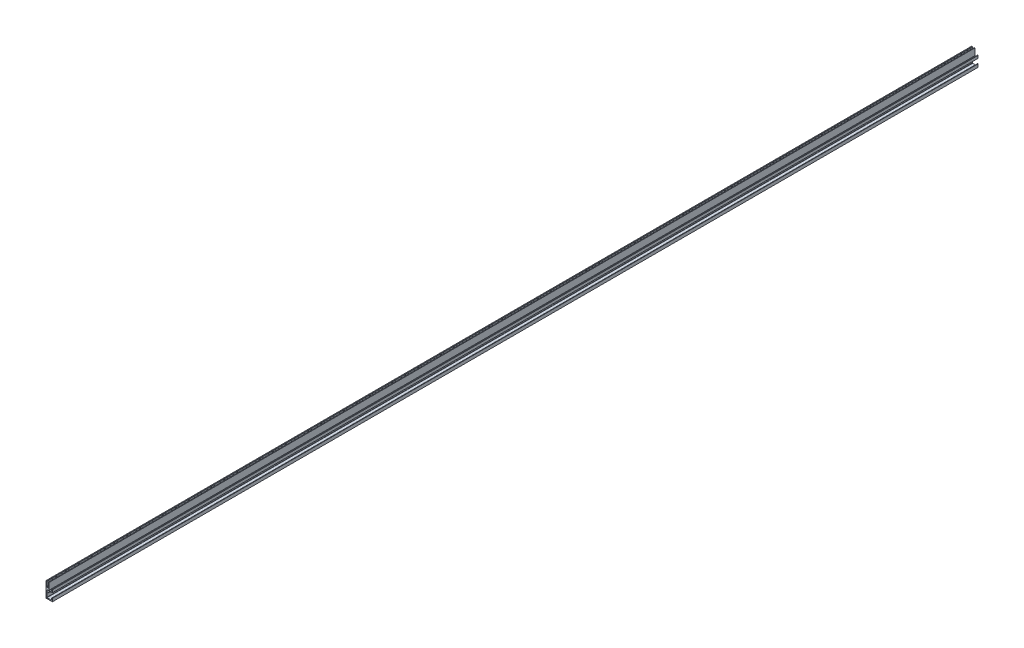
from build123d import *

# Parameters (mm, degrees)
EXTRUDE_1_DEPTH = 1058


with BuildPart() as part:
    # 草图2 → 凸台-拉伸1 (new, symmetric)
    with BuildSketch(Plane.XY):
        with BuildLine():
            Line((14.484958611, 7.149447031), (13.704975481, 7.149447031))
            ThreePointArc((13.704975481, 7.149447031), (13.280736974, 6.973721688), (13.105011631, 6.549483181))
            Line((13.105011631, 6.549483181), (13.105011631, 2.269839045))
            ThreePointArc((13.105011631, 2.269839045), (13.06986594, 2.184990722), (12.985017102, 2.149846275))
            Line((12.985017102, 2.149846275), (2.5, 2.15))
            ThreePointArc((2.5, 2.15), (2.146446609, 2.296446609), (2, 2.65))
            Line((2, 2.65), (2, 9.75))
            ThreePointArc((2, 9.75), (1.75, 10), (2, 10.25))
            Line((2, 10.25), (2, 17.35))
            ThreePointArc((2, 17.35), (2.146446609, 17.703553391), (2.5, 17.85))
            Line((2.5, 17.85), (14.604187277, 17.85))
            Line((14.604187277, 17.85), (14.604187277, 23.829737701))
            ThreePointArc((14.604187277, 23.829737701), (14.569042208, 23.914585402), (14.484194507, 23.949730471))
            Line((14.484194507, 23.949730471), (13.704211377, 23.949730471))
            ThreePointArc((13.704211377, 23.949730471), (13.27997287, 23.774005128), (13.104247527, 23.349766621))
            Line((13.104247527, 23.349766621), (13.104247527, 19.46999277))
            ThreePointArc((13.104247527, 19.46999277), (13.069102458, 19.385145069), (12.984254757, 19.35))
            Line((12.984254757, 19.35), (7.2, 19.35))
            Line((7.2, 19.35), (7.2, 34.798393128))
            Line((7.2, 34.798393128), (6, 34.798393128))
            ThreePointArc((6, 34.798393128), (5.858578644, 34.739814485), (5.8, 34.598393128))
            Line((5.8, 34.598393128), (5.8, 33.098393128))
            ThreePointArc((5.8, 33.098393128), (5.7, 32.998393128), (5.8, 32.898393128))
            Line((5.8, 32.898393128), (5.8, 23.812239282))
            ThreePointArc((5.8, 23.812239282), (5.507106781, 23.105132501), (4.8, 22.812239282))
            Line((4.8, 22.812239282), (2.8, 22.812239282))
            ThreePointArc((2.8, 22.812239282), (2.092893219, 23.105132501), (1.8, 23.812239282))
            Line((1.8, 23.812239282), (1.8, 32.898393128))
            ThreePointArc((1.8, 32.898393128), (1.9, 32.998393128), (1.8, 33.098393128))
            Line((1.8, 33.098393128), (1.8, 34.598393128))
            ThreePointArc((1.8, 34.598393128), (1.741421356, 34.739814485), (1.6, 34.798393128))
            Line((1.6, 34.798393128), (0, 34.798393128))
            Line((0, 34.798393128), (0, 0))
            Line((0, 0), (14.6, 0))
            Line((14.6, 0), (14.604951381, 7.029454261))
            ThreePointArc((14.604951381, 7.029454261), (14.569806312, 7.114301962), (14.484958611, 7.149447031))
        make_face()
    extrude(amount=EXTRUDE_1_DEPTH, both=True)


solid = part.part
